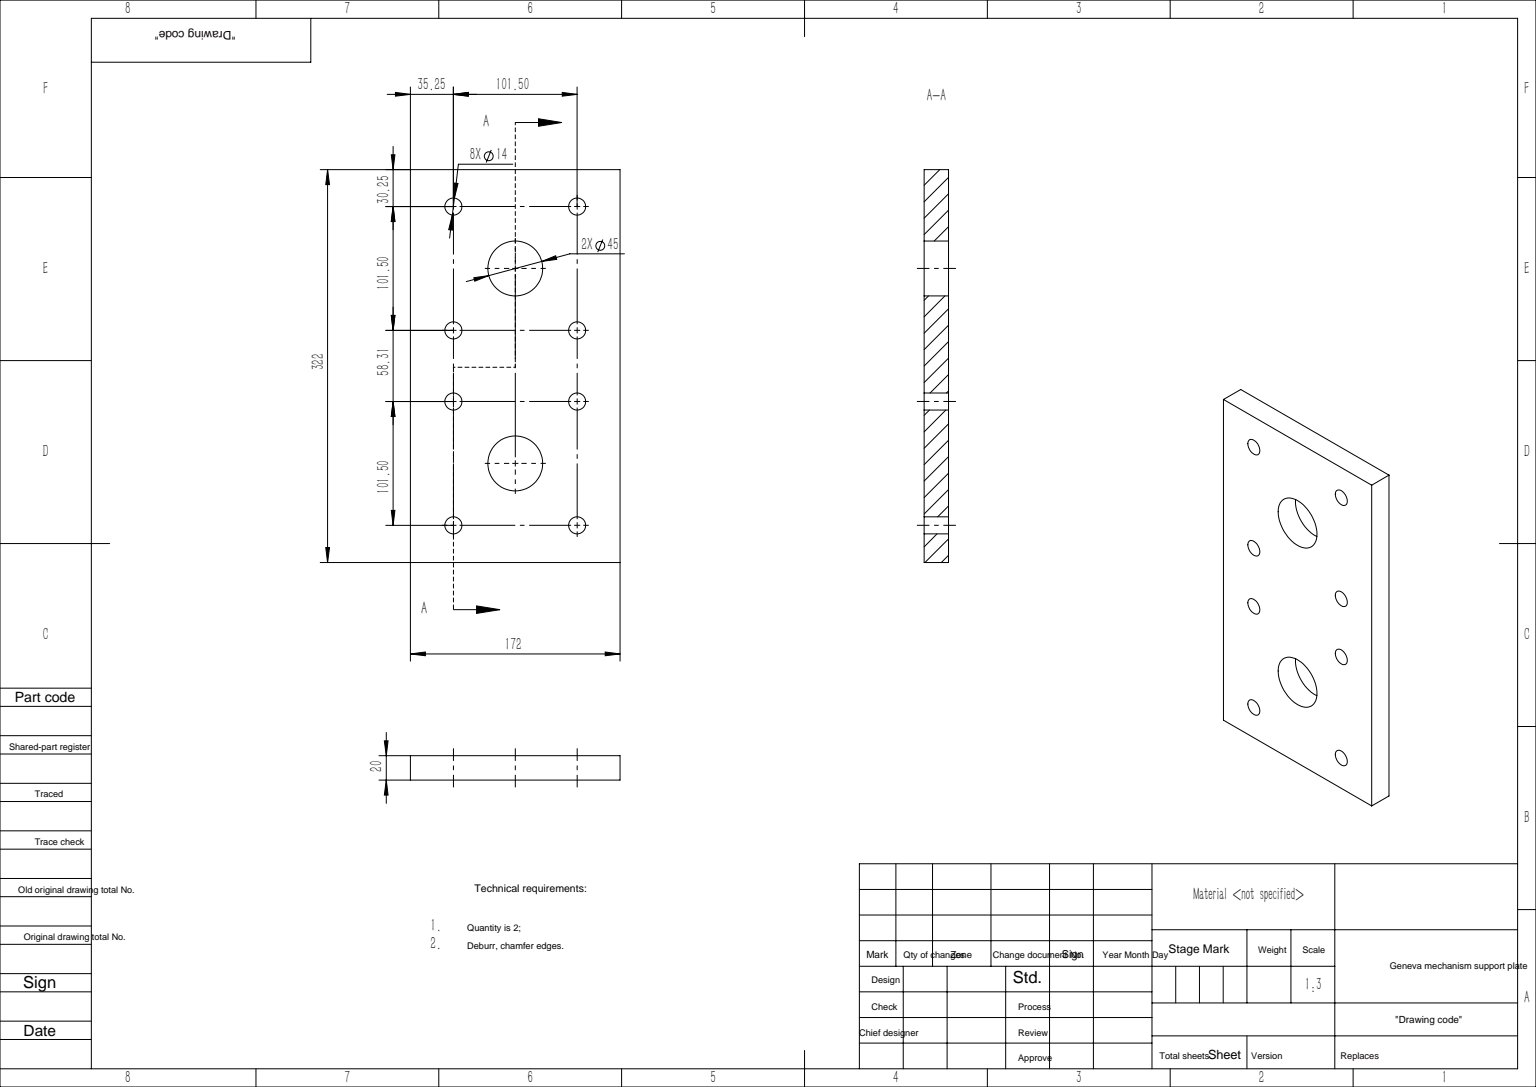
from build123d import *

# Parameters (mm, degrees)
SKETCH_1_W          = 172
SKETCH_1_H          = 322
EXTRUDE_1_DEPTH     = 20
SKETCH_3_R          = 22.5
SKETCH_3_R_2        = 7
CUT_EXTRUDE_1_DEPTH = 184.621894119


with BuildPart() as part:
    # 草图1 → 凸台-拉伸1 (new body)
    with BuildSketch(Plane.XY):
        Rectangle(SKETCH_1_W, SKETCH_1_H)
    extrude(amount=EXTRUDE_1_DEPTH)

    # 草图3 → 切除-拉伸1 (cut, through all)
    with BuildSketch(Plane(origin=(0, 0, 0), x_dir=(-1, 0, 0), z_dir=(0, 0, -1))):
        with Locations((0, 80)):
            Circle(SKETCH_3_R)
        with Locations((-50.75, 130.75)):
            Circle(SKETCH_3_R_2)
        with Locations((50.75, 130.75)):
            Circle(SKETCH_3_R_2)
        with Locations((-50.75, 29.25)):
            Circle(SKETCH_3_R_2)
        with Locations((50.75, 29.25)):
            Circle(SKETCH_3_R_2)
        with Locations((0, -79.81)):
            Circle(SKETCH_3_R)
        with Locations((-50.75, -29.06)):
            Circle(SKETCH_3_R_2)
        with Locations((50.75, -29.06)):
            Circle(SKETCH_3_R_2)
        with Locations((50.75, -130.56)):
            Circle(SKETCH_3_R_2)
        with Locations((-50.75, -130.56)):
            Circle(SKETCH_3_R_2)
    extrude(amount=-CUT_EXTRUDE_1_DEPTH, mode=Mode.SUBTRACT)


solid = part.part
